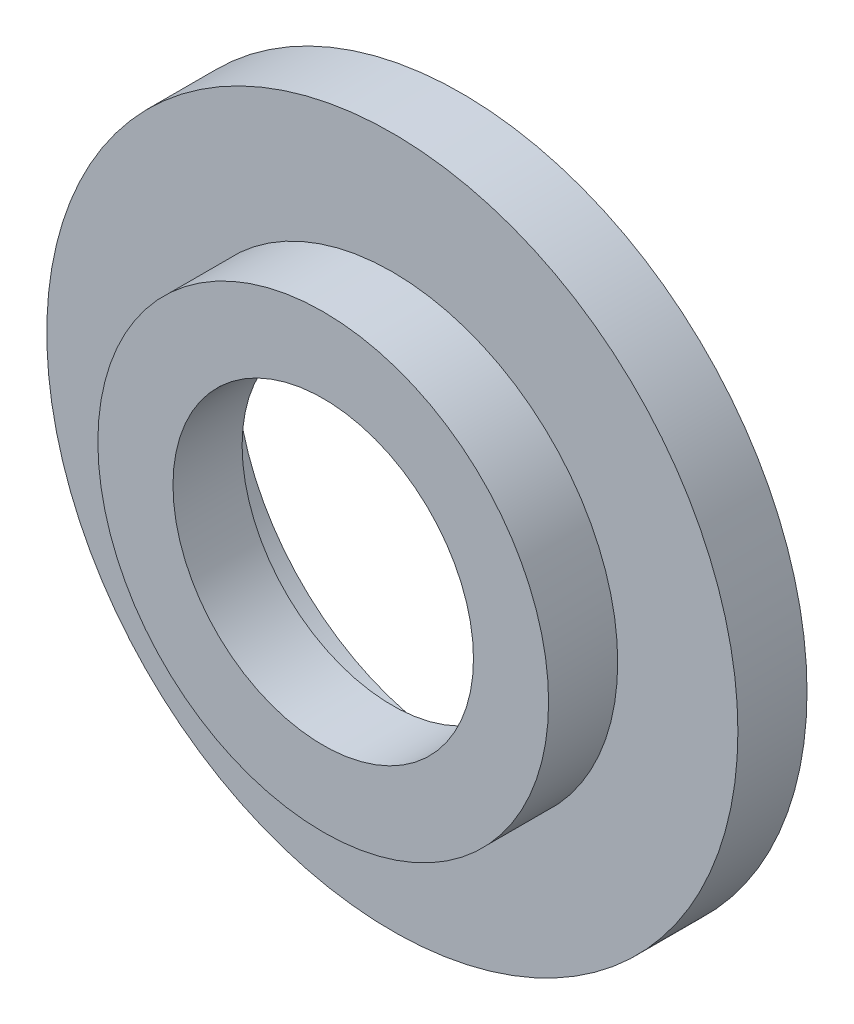
SolidWorks part; units mm, degrees
ref_plane "前视基准面" through (0, 0, 0) normal (0, 0, 1) x (1, 0, 0)
ref_plane "上视基准面" through (0, 0, 0) normal (0, 1, 0) x (1, 0, 0)
ref_plane "右视基准面" through (0, 0, 0) normal (1, 0, 0) x (0, 0, -1)
other "Configuration Table"
sketch "草图1" plane through (0, 0, 0) normal (0, 0, 1) x (1, 0, 0)
  line L0 (-82.5233, 0) -> (110.0682, 0) construction
  circle A0 centre (0, 0) radius 7.5
  circle A1 centre (0, 0) radius 11.5
extrude "凸台-拉伸1" add sketch "草图1" along normal blind 2.3
ref_plane "基准面1" through (0, 0, 2.3) normal (0, 0, 1) x (1, 0, 0)
sketch "草图2" plane through (0, 0, 2.3) normal (0, 0, 1) x (1, 0, 0)
  circle A0 centre (0, 0) radius 7.5
  circle A1 centre (0, 0) radius 5
extrude "凸台-拉伸2" add sketch "草图2" along normal blind 2.3 separate body
